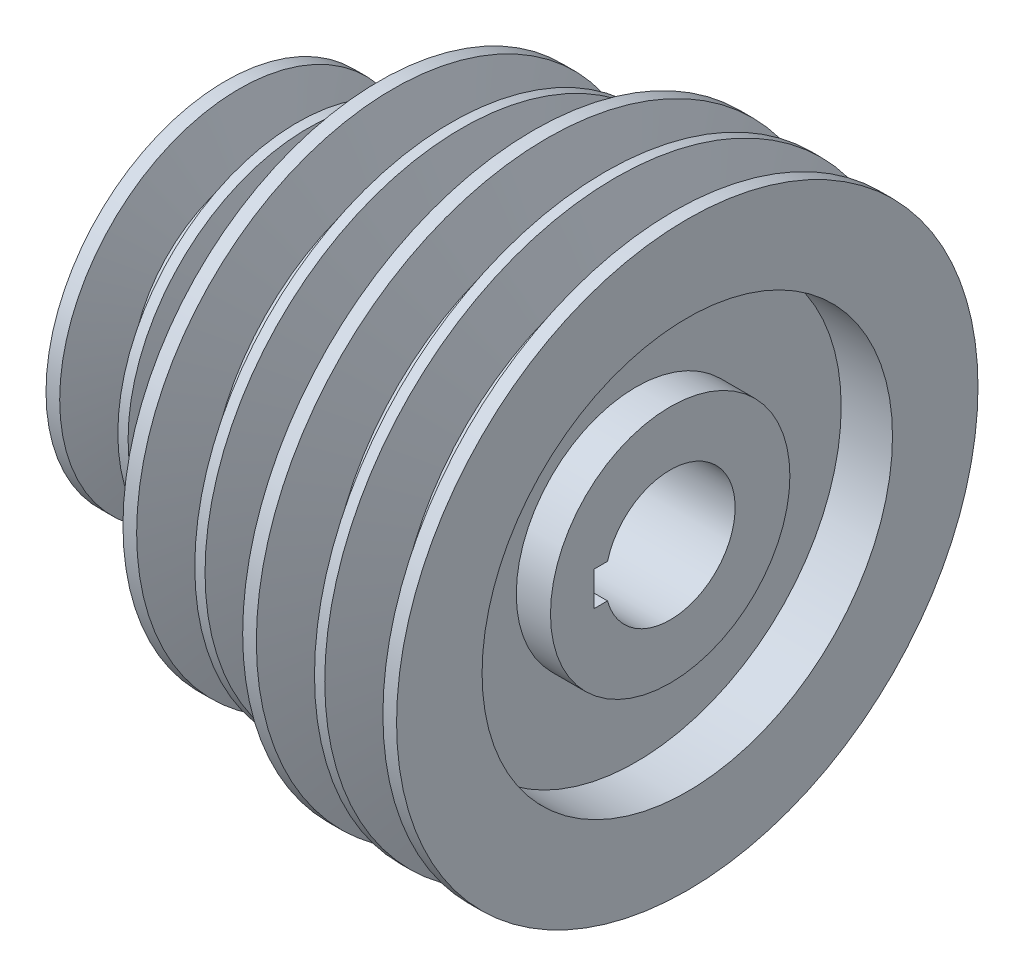
SolidWorks part; units mm, degrees
ref_plane "前视基准面" through (0, 0, 0) normal (0, 0, 1) x (1, 0, 0)
ref_plane "上视基准面" through (0, 0, 0) normal (0, 1, 0) x (1, 0, 0)
ref_plane "右视基准面" through (0, 0, 0) normal (1, 0, 0) x (0, 0, -1)
other "Configuration Table"
sketch "草图1" plane through (0, 0, 0) normal (0, 0, 1) x (1, 0, 0)
  line L0 (-46.2349, 0) -> (93.4535, 0) construction
  line L1 (0, 26) -> (0, 52.5)
  line L2 (0, 52.5) -> (4, 52.5)
  line L3 (4, 52.5) -> (8.8917, 36.5)
  line L4 (8.8917, 36.5) -> (16.1083, 36.5)
  line L5 (16.1083, 36.5) -> (21, 52.5)
  line L6 (21, 52.5) -> (24, 52.5)
  line L7 (24, 52.5) -> (28.8917, 36.5)
  line L8 (28.8917, 36.5) -> (36.1083, 36.5)
  line L9 (36.1083, 36.5) -> (41, 52.5)
  line L10 (41, 52.5) -> (45, 52.5)
  line L11 (45, 52.5) -> (45, 75)
  line L12 (45, 75) -> (49, 75)
  line L13 (49, 75) -> (53.8917, 59)
  line L14 (53.8917, 59) -> (61.1083, 59)
  line L15 (61.1083, 59) -> (66, 75)
  line L16 (66, 75) -> (69, 75)
  line L17 (69, 75) -> (73.8917, 59)
  line L18 (73.8917, 59) -> (81.1083, 59)
  line L19 (81.1083, 59) -> (86, 75)
  line L20 (86, 75) -> (90, 75)
  line L21 (90, 75) -> (90, 85)
  line L22 (90, 85) -> (94, 85)
  line L23 (94, 85) -> (98.8917, 69)
  line L24 (98.8917, 69) -> (106.1083, 69)
  line L25 (106.1083, 69) -> (111, 85)
  line L26 (111, 85) -> (114, 85)
  line L27 (114, 85) -> (118.8917, 69)
  line L28 (118.8917, 69) -> (126.1083, 69)
  line L29 (126.1083, 69) -> (131, 85)
  line L30 (131, 85) -> (135, 85)
  line L31 (135, 85) -> (135, 60)
  line L32 (135, 60) -> (120, 60)
  line L33 (120, 60) -> (120, 35)
  line L34 (120, 35) -> (130, 35)
  line L35 (130, 35) -> (130, 19)
  line L36 (130, 19) -> (30, 19)
  line L37 (30, 19) -> (30, 26)
  line L38 (30, 26) -> (0, 26)
  dimension "D1" = 30
  dimension "D2" = 52
  dimension "D3" = 105
  dimension "D4" = 150
  dimension "D5" = 38
  dimension "D6" = 70
  dimension "D7" = 120
  dimension "D8" = 170
  dimension "D9" = 34
  dimension "D10" = 34
  dimension "D11" = 34
  dimension "D12" = 17
  dimension "D13" = 17
  dimension "D14" = 17
  dimension "D15" = 17
  dimension "D16" = 17
  dimension "D17" = 17
  dimension "D18" = 4
  dimension "D19" = 16
  dimension "D20" = 16
  dimension "D21" = 4
  dimension "D22" = 45
  dimension "D23" = 107
  dimension "D24" = 4
  dimension "D25" = 16
  dimension "D26" = 16
  dimension "D27" = 150
  dimension "D28" = 105
  dimension "D29" = 105
  dimension "D30" = 150
  dimension "D31" = 170
  dimension "D32" = 170
  dimension "D33" = 3
  dimension "D34" = 4
  dimension "D35" = 4
  dimension "D36" = 4
  dimension "D37" = 16
  dimension "D38" = 16
  dimension "D39" = 135
  dimension "D40" = 120
  dimension "D41" = 130
revolve "旋转1" add sketch "草图1" angle 360 about L0
sketch "草图5" plane through (0, 0, 0) normal (-1, 0, 0) x (0, 0, 1)
  line L0 (0, 0) -> (0, 32) construction
  point P0 (0, 32)
  point P2 (0, -32)
  dimension "D1" = 32
  dimension "D2" = 32
hole_wizard "M10 螺纹孔1" positions "草图5" profile "草图4" tap size "M10" standard "GB"
sketch "草图4" plane through (0, 32, 0) normal (0, 1, 0) x (0, 0, 1)
  line L0 (0, 0) -> (0, 27.0537)
  line L1 (0, 27.0537) -> (4.25, 24.5)
  line L2 (4.25, 24.5) -> (4.25, 0)
  line L5 (4.25, 0) -> (0, 0)
  line L10 (0, 27.0537) -> (-4.25, 24.5) construction
  line L11 (0, -6.35) -> (0, 107.95) construction
  dimension "螺纹孔钻头直径" = 8.5
  dimension "螺纹孔钻头深度" = 24.5
  dimension "导头角度" = 118
cosmetic thread "孔螺纹线1" parameters "D1"=20, "D2"=10
cosmetic thread "孔螺纹线2" parameters "D1"=20, "D2"=10
sketch "草图6" plane through (130, 0, 0) normal (1, 0, 0) x (0, 0, -1)
  line L0 (0, 0) -> (-54.9274, 0) construction
  line L1 (-22.3, -5) -> (-18.3303, -5)
  line L2 (-22.3, -5) -> (-22.3, 5)
  line L3 (-22.3, 5) -> (-18.3303, 5)
  line L4 (-18.3303, -5) -> (-18.3303, 5)
  line L5 (-20.3152, 5) -> (-20.3152, -5) construction
  line L6 (-22.3, 0) -> (-18.3303, 0) construction
  line L7 (19, 0) -> (0, 0) construction
  circle A0 centre (0, 0) radius 19 construction
  point P0 (-20.3152, 0)
  dimension "D1" = 41.3
  dimension "D2" = 10
extrude "切除-拉伸1" cut sketch "草图6" against normal through all
